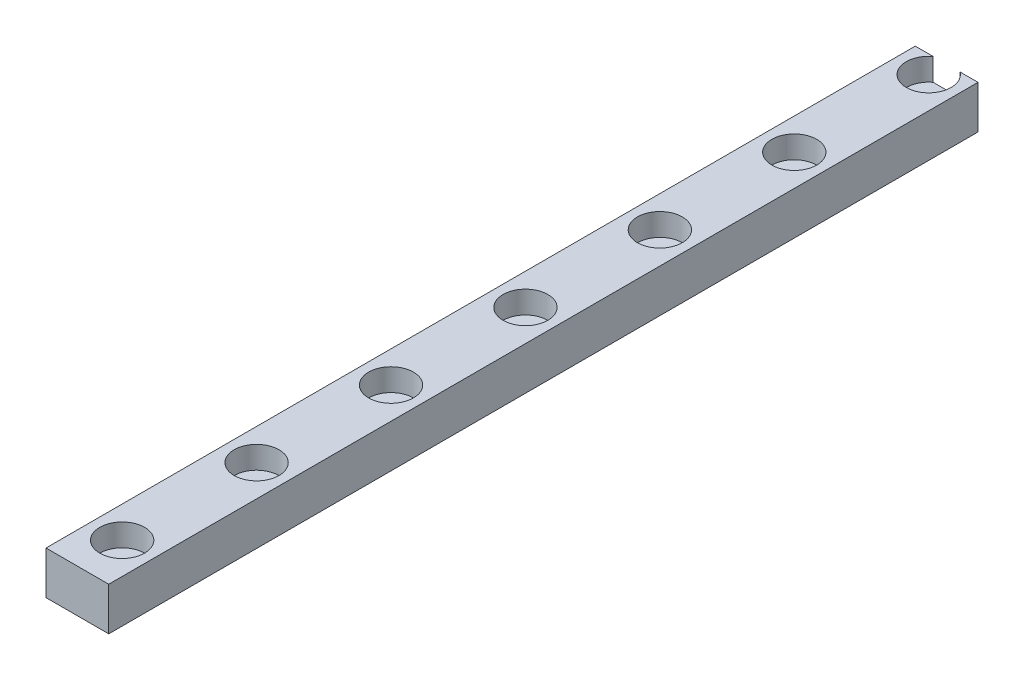
SolidWorks part; units mm, degrees
ref_plane "Front" through (0, 0, 0) normal (0, 0, 1) x (1, 0, 0)
ref_plane "Top" through (0, 0, 0) normal (0, 1, 0) x (1, 0, 0)
ref_plane "Right" through (0, 0, 0) normal (1, 0, 0) x (0, 0, -1)
sketch "Sketch1" plane through (0, 0, 0) normal (0, 0, 1) x (1, 0, 0)
  line L1 (-3.5, 2.6503) -> (3.5, 2.6503)
  line L2 (-3.5, 2.6503) -> (-3.5, -2.1497)
  line L3 (-3.5, -2.1497) -> (3.5, -2.1497)
  line L4 (3.5, 2.6503) -> (3.5, -2.1497)
  dimension "D1" = 7
  dimension "D2" = 4.8
  dimension "D3" = 3.5
extrude "Boss-Extrude1" add sketch "Sketch1" along normal blind 97 contours L1 L4 L3 L2
sketch "Sketch2" plane through (0, 2.6503, 0) normal (0, 1, 0) x (1, 0, 0)
  line L0 (-3.5, -97) -> (3.5, -97) construction
  line L1 (-3.5, -97) -> (-3.5, 0) construction
  circle A0 centre (0, -92) radius 1
  dimension "D2" = 2
  dimension "D1" = 5
  dimension "D3" = 3.5
extrude "Cut-Extrude1" cut sketch "Sketch2" against normal blind 668
sketch "Sketch3" plane through (0, 2.6503, 0) normal (0, 1, 0) x (1, 0, 0)
  circle A0 centre (0, -92) radius 2.5
  dimension "D1" = 5
extrude "Cut-Extrude2" cut sketch "Sketch3" against normal blind 2.5
pattern_linear "LPattern1" count 7 spacing 15 along (0, 0, -1) of "Cut-Extrude2", "Cut-Extrude1"
